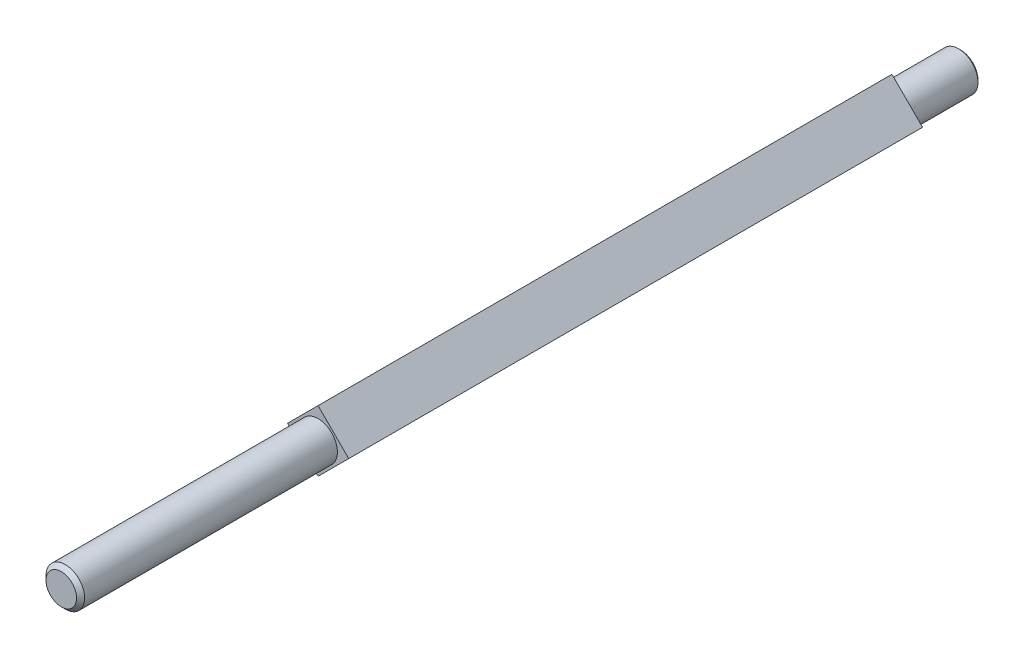
SolidWorks part; units mm, degrees
material "Q235B"
ref_plane "Front Plane" through (0, 0, 0) normal (0, 0, 1) x (1, 0, 0)
ref_plane "Top Plane" through (0, 0, 0) normal (0, 1, 0) x (1, 0, 0)
ref_plane "Right Plane" through (0, 0, 0) normal (1, 0, 0) x (0, 0, -1)
sketch "Sketch1" plane through (0, 0, 0) normal (0, 0, 1) x (1, 0, 0)
  line L0 (0, 0) -> (79.1172, 0) construction
  line L1 (0, 0) -> (0, 70.4576) construction
  line L3 (-22.6274, 0) -> (0, 22.6274)
  line L4 (-22.6274, 0) -> (0, -22.6274)
  line L5 (0, -22.6274) -> (22.6274, 0)
  line L6 (0, 22.6274) -> (22.6274, 0)
  dimension "D1" = 32
extrude "Extrude1" add sketch "Sketch1" along normal blind 664.7
sketch "Sketch2" plane through (0, 0, 0) normal (0, 1, 0) x (1, 0, 0)
  line L0 (0, 0) -> (0, -1081.7747) construction
  line L1 (0, 0) -> (-22.6274, 0) construction
  line L2 (14.2875, 0) -> (24.2875, 0)
  line L3 (14.2875, 0) -> (14.2875, -50.8)
  line L4 (14.2875, -50.8) -> (24.2875, -50.8)
  line L5 (24.2875, 0) -> (24.2875, -50.8)
  line L6 (0, -664.7) -> (-22.6274, -664.7) construction
  line L7 (14.2875, -664.7) -> (24.2875, -664.7)
  line L8 (14.2875, -664.7) -> (14.2875, -474.9)
  line L9 (14.2875, -474.9) -> (24.2875, -474.9)
  line L10 (24.2875, -664.7) -> (24.2875, -474.9)
  dimension "D1" = 28.575
  dimension "D2" = 50.8
  dimension "D3" = 10
  dimension "D4" = 424.1
revolve "Cut-Revolve1" cut sketch "Sketch2" angle 360 about L0
chamfer "Chamfer1" distance 1.5 angle 45 1 edges at (-14.2875, 0, 0)
chamfer "Chamfer2" distance 3 angle 45 1 edges at (-14.2875, 0, 664.7)
